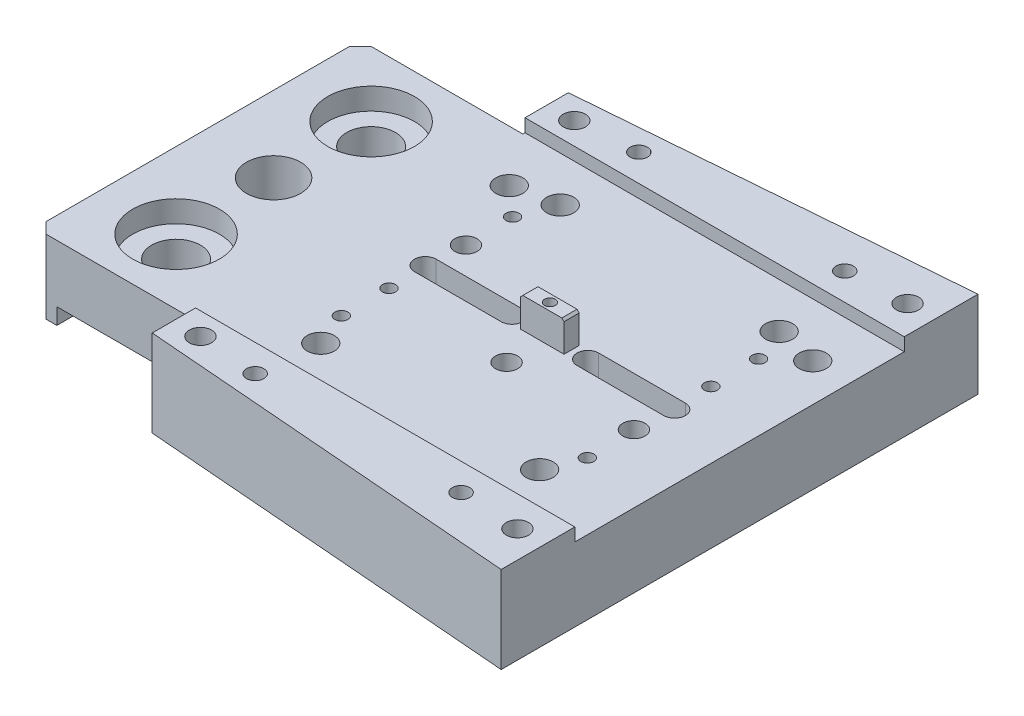
from build123d import *

# Parameters (mm, degrees)
SKETCH1_W                                            = 35
SKETCH1_H                                            = 44
BOSS_EXTRUDE1_DEPTH                                  = 4
CUT_EXTRUDE2_DEPTH                                   = 30.227555491
SKETCH15_W                                           = 30.4
SKETCH15_H                                           = 1.2
CUT_EXTRUDE6_DEPTH                                   = 42.533119315
SKETCH4_W                                            = 4
SKETCH4_H                                            = 1.4
BOSS_EXTRUDE2_DEPTH                                  = 2.8
CHAMFER1_SIZE                                        = 0.2
F_1_2_1_2_DIAMETER_HOLE1_D                           = 1
SKETCH7_R                                            = 1.25
CUT_EXTRUDE3_DEPTH                                   = 5
M3_TAPPED_HOLE1_D                                    = 2.5
SKETCH11_W                                           = 3.5
SKETCH11_H                                           = 8
CUT_EXTRUDE4_DEPTH                                   = 1
SKETCH12_R                                           = 0.5
CUT_EXTRUDE5_DEPTH                                   = 1
M2_5_TAPPED_HOLE1_D                                  = 2.05
F_1_2_1_2_DIAMETER_HOLE2_D                           = 1.2
F_1_2_1_2_DIAMETER_HOLE2_DEPTH                       = 5
F_1_2_1_2_DIAMETER_HOLE2_TIP                         = 0.360516371
M2_5_TAPPED_HOLE2_D                                  = 2.05
M3_TAPPED_HOLE2_D                                    = 2.5
CUT_EXTRUDE7_DEPTH                                   = 30.227555491
M2_5_TAPPED_HOLE3_D                                  = 2.05
M2_5_TAPPED_HOLE3_DEPTH                              = 6.5
M2_5_TAPPED_HOLE3_TIP                                = 0.615882135
M2_TAPPED_HOLE1_D                                    = 1.6
M2_TAPPED_HOLE1_DEPTH                                = 6
M2_TAPPED_HOLE1_TIP                                  = 0.480688495
SKETCH29_W                                           = 30
SKETCH29_H                                           = 6.8
BOSS_EXTRUDE3_DEPTH                                  = 15
SKETCH30_W                                           = 10
SKETCH30_H                                           = 30
CUT_EXTRUDE8_DEPTH                                   = 1.5
HOLE_SIZE_PER_SOCKET_HEAD_CAP_SCREW_TYPE_D           = 4.5
HOLE_SIZE_PER_SOCKET_HEAD_CAP_SCREW_TYPE_CBORE_D     = 8
HOLE_SIZE_PER_SOCKET_HEAD_CAP_SCREW_TYPE_CBORE_DEPTH = 2
CHAMFER3_SIZE                                        = 1
F_5_0_5_DIAMETER_HOLE1_D                             = 5


with BuildPart() as part:
    # Sketch1 → Boss-Extrude1 (new, symmetric)
    with BuildSketch(Plane(origin=(0, 0, 0), x_dir=(1, 0, 0), z_dir=(0, 1, 0))):
        Rectangle(SKETCH1_W, SKETCH1_H)
    extrude(amount=BOSS_EXTRUDE1_DEPTH, both=True)

    # Sketch3 → Cut-Extrude2 (cut, through all)
    with BuildSketch(Plane(origin=(0, 4, 0), x_dir=(1, 0, 0), z_dir=(0, 1, 0))):
        with BuildLine():
            Line((-11.5, 1), (-3.5, 1))
            ThreePointArc((-3.5, 1), (-2.5, 0), (-3.5, -1))
            Line((-3.5, -1), (-11.5, -1))
            ThreePointArc((-11.5, -1), (-12.5, 0), (-11.5, 1))
        make_face()
        with BuildLine():
            Line((3.5, 1), (11.5, 1))
            ThreePointArc((11.5, 1), (12.5, 0), (11.5, -1))
            Line((11.5, -1), (3.5, -1))
            ThreePointArc((3.5, -1), (2.5, 0), (3.5, 1))
        make_face()
    extrude(amount=-CUT_EXTRUDE2_DEPTH, mode=Mode.SUBTRACT)

    # Sketch15 → Cut-Extrude6 (cut, through all)
    with BuildSketch(Plane(origin=(17.5, 0, 0), x_dir=(0, 0, -1), z_dir=(1, 0, 0))):
        with Locations((0, 3.4)):
            Rectangle(SKETCH15_W, SKETCH15_H)
    extrude(amount=-CUT_EXTRUDE6_DEPTH, mode=Mode.SUBTRACT)

    # Sketch4 → Boss-Extrude2 (add)
    with BuildSketch(Plane(origin=(0, 2.8, 0), x_dir=(1, 0, 0), z_dir=(0, 1, 0))):
        Rectangle(SKETCH4_W, SKETCH4_H)
    extrude(amount=BOSS_EXTRUDE2_DEPTH)

    # Chamfer1
    chamfer1_edges = [part.edges().sort_by_distance(p)[0] for p in [
        (2, 5.6, 0),
        (-2, 5.6, 0),
    ]]
    chamfer(chamfer1_edges, length=CHAMFER1_SIZE)

    # Ø1.2 (1.2) Diameter Hole1 (through all)
    with Locations(Plane(origin=(0, -4, 0), x_dir=(-1, 0, 0), z_dir=(0, -1, 0))):
        with Locations((0, 0)):
            Hole(F_1_2_1_2_DIAMETER_HOLE1_D / 2)

    # Sketch7 → Cut-Extrude3 (cut)
    with BuildSketch(Plane.XZ.offset(4)):
        with Locations(Location((0, 0, 0), (0, 0, 270))):
            Circle(SKETCH7_R)
    extrude(amount=-CUT_EXTRUDE3_DEPTH, mode=Mode.SUBTRACT)

    # M3 Tapped Hole1 (through all)
    with Locations(Plane(origin=(0, -4, 0), x_dir=(-1, 0, 0), z_dir=(0, -1, 0))):
        with Locations((14, 10.25), (-14, 10.25)):
            Hole(M3_TAPPED_HOLE1_D / 2)

    # Sketch11 → Cut-Extrude4 (cut)
    with BuildSketch(Plane.XZ.offset(4)):
        with Locations((0, 2)):
            Rectangle(SKETCH11_W, SKETCH11_H)
    extrude(amount=-CUT_EXTRUDE4_DEPTH, mode=Mode.SUBTRACT)

    # Sketch12 → Cut-Extrude5 (cut)
    with BuildSketch(Plane.XZ.offset(4)):
        with Locations((-1.75, 6)):
            Circle(SKETCH12_R)
        with Locations((1.75, 6)):
            Circle(SKETCH12_R)
        with Locations((-1.75, -2)):
            Circle(SKETCH12_R)
        with Locations((1.75, -2)):
            Circle(SKETCH12_R)
    extrude(amount=-CUT_EXTRUDE5_DEPTH, mode=Mode.SUBTRACT)

    # M2.5 Tapped Hole1 (through all)
    with Locations(Plane(origin=(0, -3, 0), x_dir=(-1, 0, 0), z_dir=(0, -1, 0))):
        with Locations((0, -4)):
            Hole(M2_5_TAPPED_HOLE1_D / 2)

    # Ø1.2 (1.2) Diameter Hole2
    with Locations(Plane(origin=(0, 2.8, 0), x_dir=(1, 0, 0), z_dir=(0, 1, 0))):
        with Locations((-11.35, 7.9), (11.35, 7.9), (-11.35, -3.5), (11.35, 3.5), (11.35, -7.9), (-11.35, -7.9)):
            Hole(F_1_2_1_2_DIAMETER_HOLE2_D / 2, depth=F_1_2_1_2_DIAMETER_HOLE2_DEPTH)
            with Locations((0, 0, -(F_1_2_1_2_DIAMETER_HOLE2_DEPTH + F_1_2_1_2_DIAMETER_HOLE2_TIP / 2))):  # 118° drill point
                Cone(0, F_1_2_1_2_DIAMETER_HOLE2_D / 2, F_1_2_1_2_DIAMETER_HOLE2_TIP, mode=Mode.SUBTRACT)

    # M2.5 Tapped Hole2 (through all)
    with Locations(Plane(origin=(0, 2.8, 0), x_dir=(1, 0, 0), z_dir=(0, 1, 0))):
        with Locations((-11.25, 3.5), (11.25, -3.5)):
            Hole(M2_5_TAPPED_HOLE2_D / 2)

    # M3 Tapped Hole2 (through all)
    with Locations(Plane(origin=(0, 2.8, 0), x_dir=(1, 0, 0), z_dir=(0, 1, 0))):
        with Locations((-10.1, 11.05), (10.1, 11.05), (-10.1, -11.05), (10.1, -11.05)):
            Hole(M3_TAPPED_HOLE2_D / 2)

    # Sketch22 → Cut-Extrude7 (cut, through all)
    with BuildSketch(Plane(origin=(0, 4, 0), x_dir=(1, 0, 0), z_dir=(0, 1, 0))):
        Polygon((-17.5, -19.2), (-17.5, -22), (17.5, -22), align=None)
        Polygon((-17.5, 19.2), (-17.5, 22), (17.5, 22), align=None)
    extrude(amount=-CUT_EXTRUDE7_DEPTH, mode=Mode.SUBTRACT)

    # M2.5 Tapped Hole3
    with Locations(Plane(origin=(0, 4, 0), x_dir=(1, 0, 0), z_dir=(0, 1, 0))):
        with Locations((-15, -17.25), (-15, 17.25), (15, 18), (15, -18)):
            Hole(M2_5_TAPPED_HOLE3_D / 2, depth=M2_5_TAPPED_HOLE3_DEPTH)
            with Locations((0, 0, -(M2_5_TAPPED_HOLE3_DEPTH + M2_5_TAPPED_HOLE3_TIP / 2))):  # 118° drill point
                Cone(0, M2_5_TAPPED_HOLE3_D / 2, M2_5_TAPPED_HOLE3_TIP, mode=Mode.SUBTRACT)

    # M2 Tapped Hole1
    with Locations(Plane(origin=(0, 4, 0), x_dir=(1, 0, 0), z_dir=(0, 1, 0))):
        with Locations((-9.5, 17.7), (9.5, 17.7), (9.5, -17.7), (-9.5, -17.7)):
            Hole(M2_TAPPED_HOLE1_D / 2, depth=M2_TAPPED_HOLE1_DEPTH)
            with Locations((0, 0, -(M2_TAPPED_HOLE1_DEPTH + M2_TAPPED_HOLE1_TIP / 2))):  # 118° drill point
                Cone(0, M2_TAPPED_HOLE1_D / 2, M2_TAPPED_HOLE1_TIP, mode=Mode.SUBTRACT)

    # Sketch29 → Boss-Extrude3 (add)
    with BuildSketch(Plane.ZY.offset(17.5)):
        with Locations((0, -0.6)):
            Rectangle(SKETCH29_W, SKETCH29_H)
    extrude(amount=BOSS_EXTRUDE3_DEPTH)

    # Sketch30 → Cut-Extrude8 (cut)
    with BuildSketch(Plane.XZ.offset(4)):
        with Locations((-25.5, 0)):
            Rectangle(SKETCH30_W, SKETCH30_H)
    extrude(amount=-CUT_EXTRUDE8_DEPTH, mode=Mode.SUBTRACT)

    # Hole size per socket head cap screw type1 (through all)
    with Locations(Plane(origin=(0, 2.8, 0), x_dir=(1, 0, 0), z_dir=(0, 1, 0))):
        with Locations((-25.5, 9), (-25.5, -9)):
            CounterBoreHole(HOLE_SIZE_PER_SOCKET_HEAD_CAP_SCREW_TYPE_D / 2, HOLE_SIZE_PER_SOCKET_HEAD_CAP_SCREW_TYPE_CBORE_D / 2, HOLE_SIZE_PER_SOCKET_HEAD_CAP_SCREW_TYPE_CBORE_DEPTH)

    # Chamfer3
    chamfer3_edges = [part.edges().sort_by_distance(p)[0] for p in [
        (-32.5, -0.6, 15),
        (-32.5, -0.6, -15),
    ]]
    chamfer(chamfer3_edges, length=CHAMFER3_SIZE)

    # Ø5.0 (5) Diameter Hole1 (through all)
    with Locations(Plane(origin=(0, 2.8, 0), x_dir=(1, 0, 0), z_dir=(0, 1, 0))):
        with Locations((-25.5, 0)):
            Hole(F_5_0_5_DIAMETER_HOLE1_D / 2)


solid = part.part
